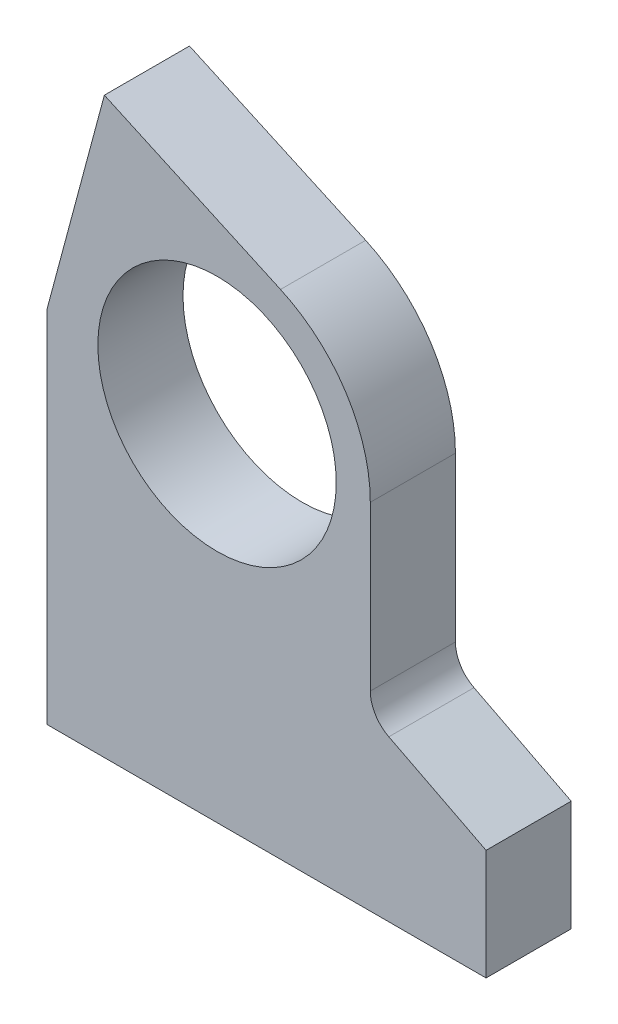
from build123d import *

# Parameters (mm, degrees)
SKETCH_1_R      = 35
EXTRUDE_1_DEPTH = 25


with BuildPart() as part:
    # 草图1 → 凸台-拉伸1 (new body)
    with BuildSketch(Plane.XY):
        with BuildLine():
            Line((129, 0), (129, 10))
            Line((129, 10), (100.448181422, 24.59601507))
            ThreePointArc((100.448181422, 24.59601507), (96.470105928, 28.280717759), (95, 33.5))
            Line((95, 33.5), (95, 81.5))
            ThreePointArc((95, 81.5), (87.840181999, 105.854067962), (68.639083275, 122.458327293))
            Line((68.639083275, 122.458327293), (16.907594042, 146))
            Line((16.907594042, 146), (0, 82.9))
            Line((0, 82.9), (0, -22.47))
            Line((0, -22.47), (129, -22.47))
            Line((129, -22.47), (129, 0))
        make_face()
        with Locations((50, 81.5)):
            Circle(SKETCH_1_R, mode=Mode.SUBTRACT)
    extrude(amount=EXTRUDE_1_DEPTH)


solid = part.part
